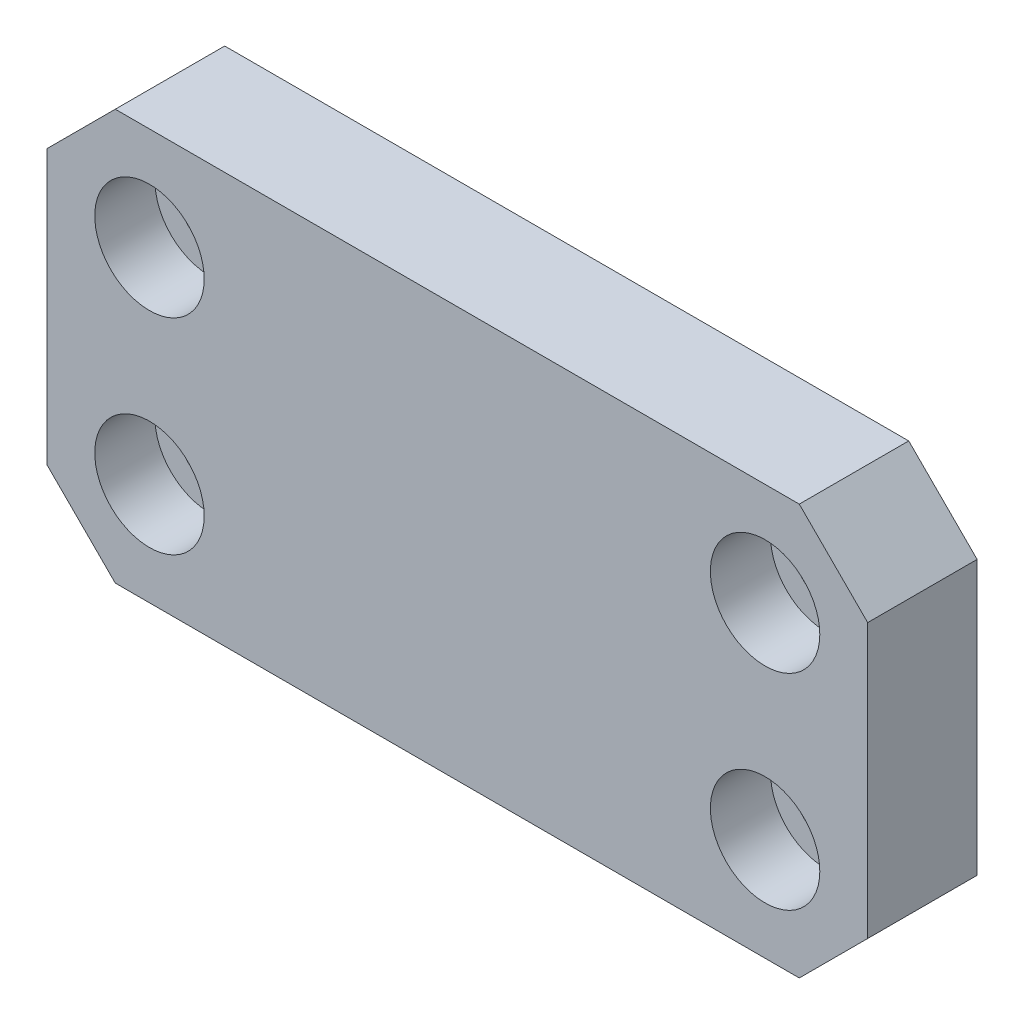
SolidWorks part; units mm, degrees
material "AL6061"
ref_plane "Front Plane" through (0, 0, 0) normal (0, 0, 1) x (1, 0, 0)
ref_plane "Top Plane" through (0, 0, 0) normal (0, 1, 0) x (1, 0, 0)
ref_plane "Right Plane" through (0, 0, 0) normal (1, 0, 0) x (0, 0, -1)
sketch "Sketch1" plane through (0, 0, 0) normal (0, 0, 1) x (1, 0, 0)
  line L1 (-30, 15) -> (30, 15)
  line L2 (-30, 15) -> (-30, -15)
  line L3 (-30, -15) -> (30, -15)
  line L4 (30, 15) -> (30, -15)
  line L5 (-30, 15) -> (30, -15) construction
  line L6 (-30, -15) -> (30, 15) construction
  point P0 (0, 0)
  dimension "D1" = 30
  dimension "D2" = 60
extrude "Boss-Extrude1" add sketch "Sketch1" along normal blind 8
hole_wizard "CBORE for M4 Hex Socket Head Cap Screw1" positions "Sketch2" profile "Sketch3" counterbore size "M4" standard "ISO" end condition through all
sketch "Sketch2" plane through (0, 0, 8) normal (0, 0, 1) x (1, 0, 0)
  line L0 (-30, 0) -> (30, 0) construction
  line L1 (-30, 15) -> (-30, -15) construction
  line L2 (30, -15) -> (30, 15) construction
  line L5 (0, 15) -> (0, -15) construction
  line L6 (30, 15) -> (-30, 15) construction
  line L7 (-30, -15) -> (30, -15) construction
  point P18 (-22.5, 7.5)
  point P21 (-22.5, -7.5)
  point P22 (22.5, -7.5)
  point P23 (22.5, 7.5)
  dimension "D1" = 15
  dimension "D2" = 45
sketch "Sketch3" plane through (22.5, 7.5, 8) normal (1, 0, 0) x (0, -1, 0)
  line L0 (0, 0) -> (0, 8)
  line L1 (0, 8) -> (2.25, 8)
  line L3 (2.25, 8) -> (2.25, 4.4)
  line L4 (2.25, 4.4) -> (4, 4.4)
  line L5 (4, 4.4) -> (4, 0)
  line L7 (4, 0) -> (0, 0)
  line L11 (0, -6.35) -> (0, 107.95) construction
  dimension "通孔孔直径" = 4.5
  dimension "通孔孔深度" = 8
  dimension "柱形沉头孔直径" = 8
  dimension "柱形沉头孔深度" = 4.4
chamfer "Chamfer1" distance 5 angle 45 4 edges at (30, 15, 4) (30, -15, 4) (-30, -15, 4) (-30, 15, 4)
